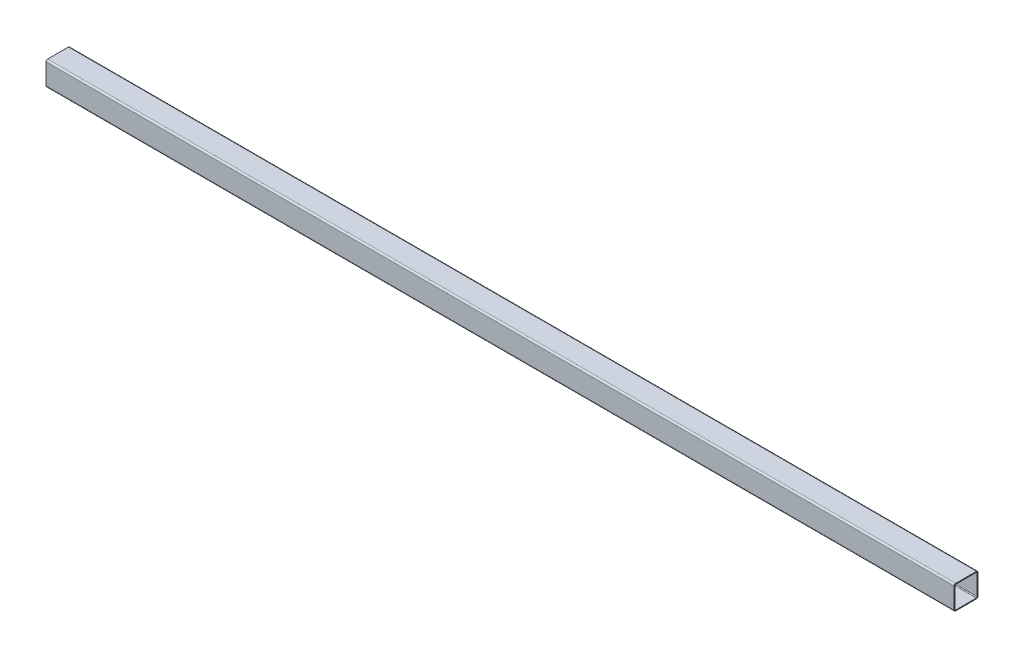
SolidWorks part; units mm, degrees
ref_plane "前视基准面" through (0, 0, 0) normal (0, 0, 1) x (1, 0, 0)
ref_plane "上视基准面" through (0, 0, 0) normal (0, 1, 0) x (1, 0, 0)
ref_plane "右视基准面" through (0, 0, 0) normal (1, 0, 0) x (0, 0, -1)
sketch "草图1" plane through (0, 0, 0) normal (0, 0, 1) x (1, 0, 0)
  line L0 (-2850, 0) -> (2850, 0)
  point P4 (0, 0)
  dimension "D1" = 5700
other "Gb／6728-1986方形空心型钢 150 X 150 X 5(1)"
ref_plane "基准面1" through (-2850, 0, 0) normal (1, 0, 0) x (0, 1, 0)
sketch "Sketch1" plane through (-2850, 0, 0) normal (1, 0, 0) x (0, 1, 0)
  line L0 (-65, -70) -> (65, -70)
  line L1 (-70, -65) -> (-70, 65)
  line L2 (65, 70) -> (-65, 70)
  line L3 (70, 65) -> (70, -65)
  line L4 (-65, -75) -> (65, -75)
  line L5 (-75, -65) -> (-75, 65)
  line L6 (65, 75) -> (-65, 75)
  line L7 (75, 65) -> (75, -65)
  arc A0 (75, 65) -> (65, 75) centre (65, 65) ccw
  arc A1 (65, -75) -> (75, -65) centre (65, -65) ccw
  arc A2 (-75, -65) -> (-65, -75) centre (-65, -65) ccw
  arc A3 (-65, 75) -> (-75, 65) centre (-65, 65) ccw
  arc A4 (-65, 70) -> (-70, 65) centre (-65, 65) ccw
  arc A5 (70, 65) -> (65, 70) centre (65, 65) ccw
  arc A6 (65, -70) -> (70, -65) centre (65, -65) ccw
  arc A7 (-70, -65) -> (-65, -70) centre (-65, -65) ccw
  point P0 (-75, 0)
  point P1 (75, 0)
  point P2 (0, 75)
  point P3 (0, -75)
  point P4 (0, 0)
  point P5 (-75, -75)
  point P6 (75, -75)
  point P7 (75, 75)
  point P8 (-75, 75)
  point P33 (0, 0)
  dimension "D1" = 10
  dimension "Thickness" = 5
  dimension "V_leg" = 150
